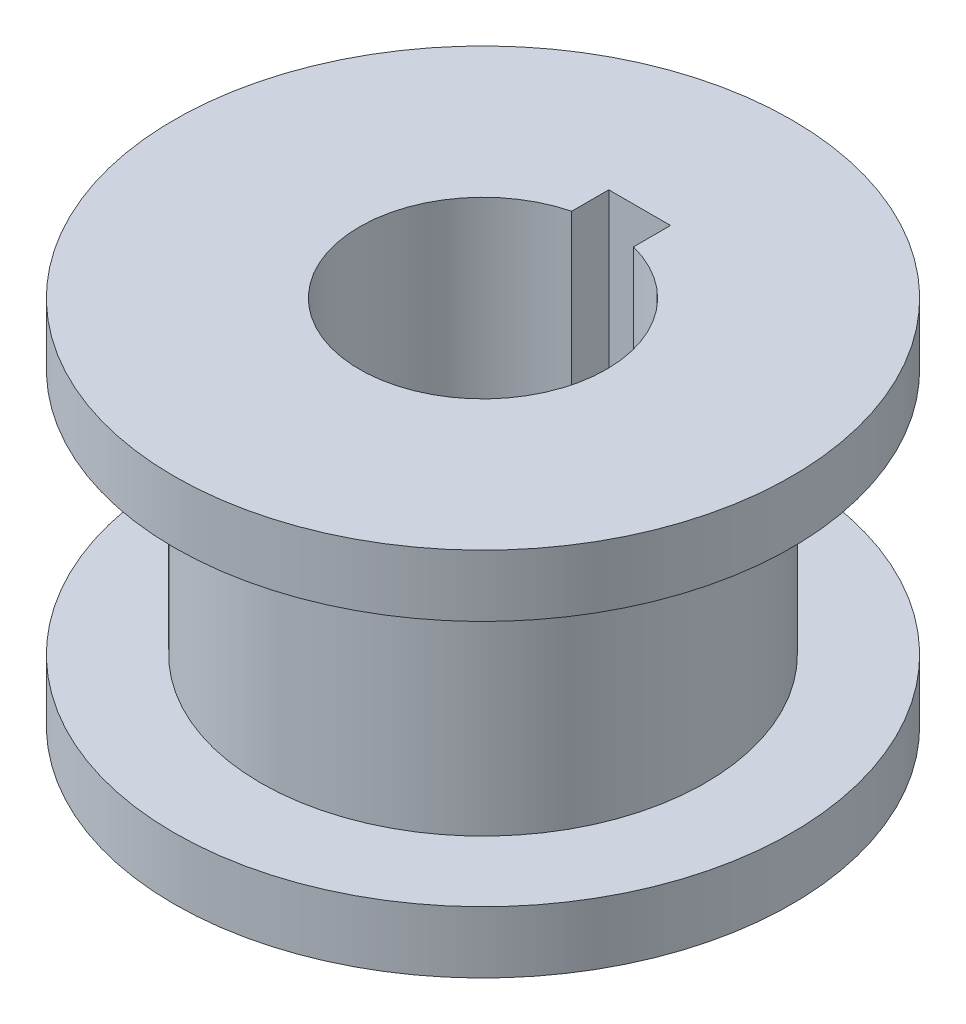
SolidWorks part; units mm, degrees
ref_plane "Front Plane" through (0, 0, 0) normal (0, 0, 1) x (1, 0, 0)
ref_plane "Top Plane" through (0, 0, 0) normal (0, 1, 0) x (1, 0, 0)
ref_plane "Right Plane" through (0, 0, 0) normal (1, 0, 0) x (0, 0, -1)
sketch "Sketch1" plane through (0, 0, 0) normal (0, 0, 1) x (1, 0, 0)
  line L0 (0, 76.7586) -> (0, -32.738) construction
  line L1 (-10, 0) -> (-10, -30)
  line L2 (-10, -30) -> (-25, -30)
  line L3 (-25, -30) -> (-25, -25)
  line L4 (-25, -25) -> (-18, -25)
  line L5 (-18, -25) -> (-18, -5)
  line L6 (-18, -5) -> (-25, -5)
  line L7 (-25, -5) -> (-25, 0)
  line L8 (-25, 0) -> (-10, 0)
  line L9 (0, 0) -> (-73.7995, 0) construction
  dimension "D1" = 10
  dimension "D2" = 25
  dimension "D3" = 18
  dimension "D4" = 5
  dimension "D5" = 20
revolve "Revolve1" add sketch "Sketch1" angle 360 about L0
sketch "Sketch2" plane through (0, 0, 0) normal (0, 1, 0) x (1, 0, 0)
  line L0 (0, 20.0252) -> (0, -7.5886) construction
  line L1 (-2.5, 12.6825) -> (-2.5, 9.6825)
  line L2 (-2.5, 12.6825) -> (2.5, 12.6825)
  line L3 (2.5, 12.6825) -> (2.5, 9.6825)
  circle A0 centre (0, 0) radius 10 construction
  arc A1 (2.5, 9.6825) -> (-2.5, 9.6825) centre (0, 0) ccw
  dimension "D1" = 3
  dimension "D2" = 5
extrude "Cut-Extrude1" cut sketch "Sketch2" against normal through all
